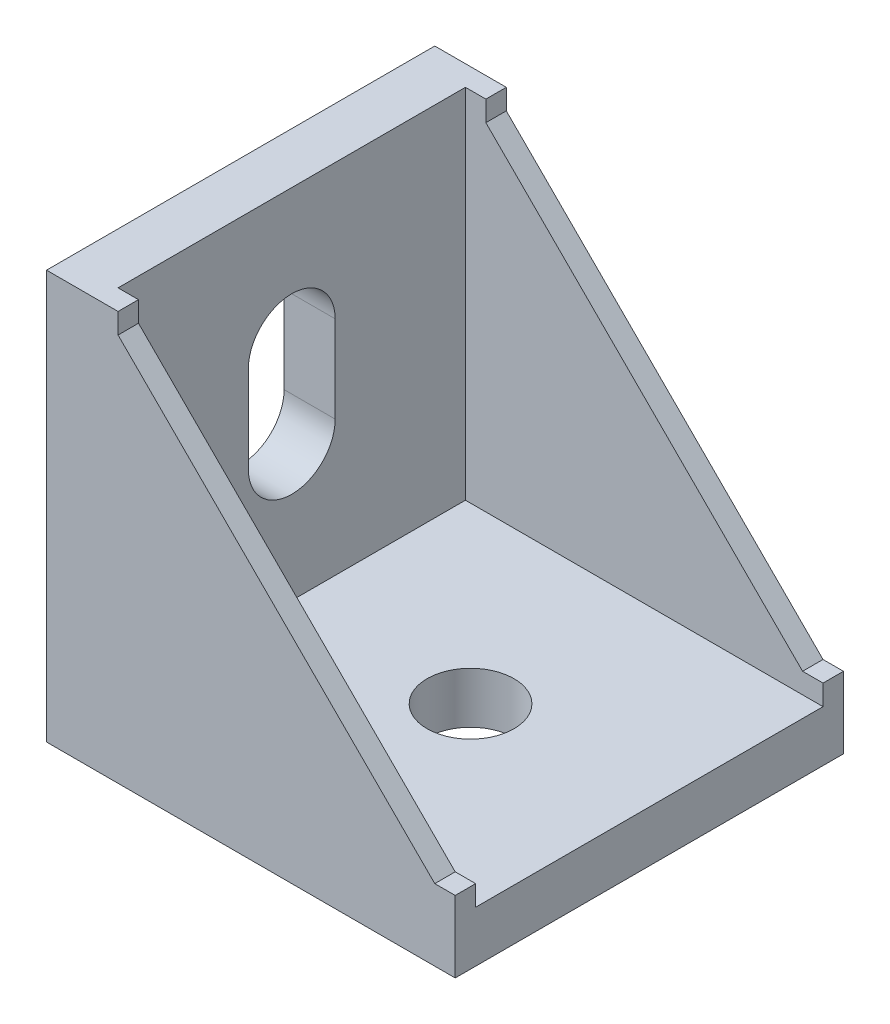
from build123d import *

# Parameters (mm, degrees)
BOSS_EXTRUDE1_DEPTH = 38
BOSS_EXTRUDE2_DEPTH = 2
BOSS_EXTRUDE3_DEPTH = 2
SKETCH4_R           = 4.25
CUT_EXTRUDE1_DEPTH  = 66.337584896
CUT_EXTRUDE2_DEPTH  = 69.14690015


with BuildPart() as part:
    # Sketch1 → Boss-Extrude1 (new body)
    with BuildSketch(Plane.XY):
        Polygon((0, 0), (40, 0), (40, 5), (5, 5), (5, 40), (0, 40), align=None)
    extrude(amount=BOSS_EXTRUDE1_DEPTH)

    # Sketch2 → Boss-Extrude2 (add)
    with BuildSketch(Plane.XY.offset(38)):
        Polygon((7, 40), (7, 38), (38, 7), (40, 7), (40, 5), (5, 5), (5, 40), align=None)
    extrude(amount=-BOSS_EXTRUDE2_DEPTH)

    # Sketch3 → Boss-Extrude3 (add)
    with BuildSketch(Plane(origin=(0, 0, 0), x_dir=(-1, 0, 0), z_dir=(0, 0, -1))):
        Polygon((-38, 7), (-7, 38), (-7, 40), (-5, 40), (-5, 5), (-40, 5), (-40, 7), align=None)
    extrude(amount=-BOSS_EXTRUDE3_DEPTH)

    # Sketch4 → Cut-Extrude1 (cut, through all)
    with BuildSketch(Plane(origin=(0, 5, 0), x_dir=(1, 0, 0), z_dir=(0, 1, 0))):
        with Locations(Location((22.5, -19, 0), (0, 0, 270))):
            Circle(SKETCH4_R)
    extrude(amount=-CUT_EXTRUDE1_DEPTH, mode=Mode.SUBTRACT)

    # Sketch5 → Cut-Extrude2 (cut, through all)
    with BuildSketch(Plane.ZY):
        with BuildLine():
            Line((14.75, 22.5), (14.75, 18.25))
            ThreePointArc((14.75, 18.25), (19, 14), (23.25, 18.25))
            Line((23.25, 18.25), (23.25, 26.75))
            ThreePointArc((23.25, 26.75), (19, 31), (14.75, 26.75))
            Line((14.75, 26.75), (14.75, 22.5))
        make_face()
    extrude(amount=-CUT_EXTRUDE2_DEPTH, mode=Mode.SUBTRACT)


solid = part.part
